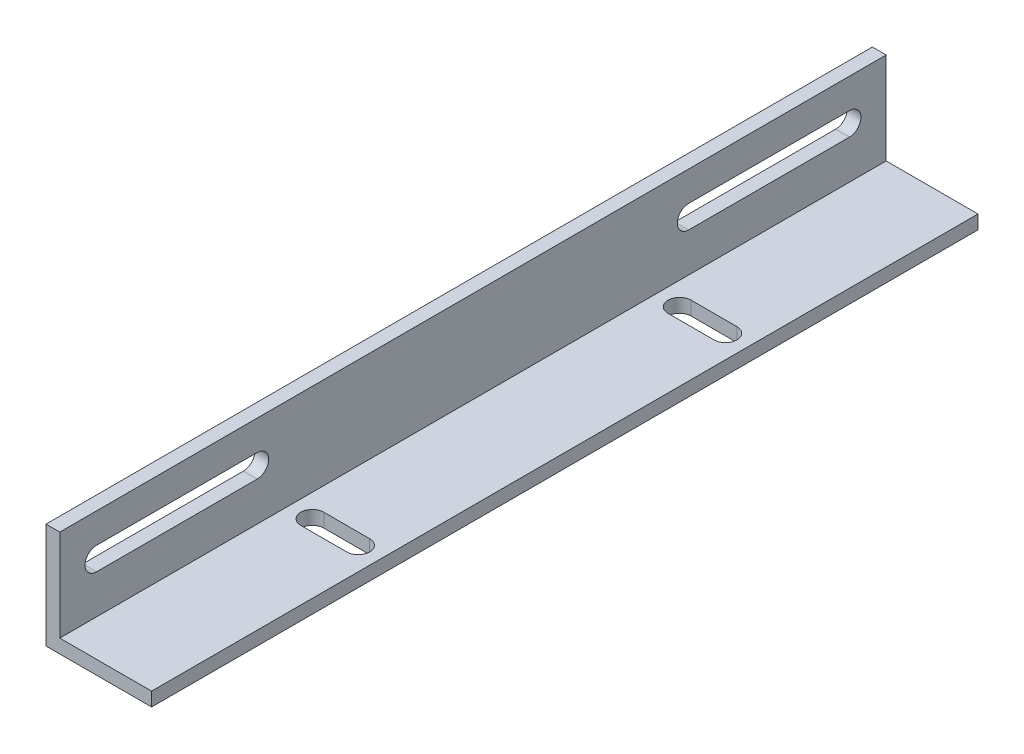
SolidWorks part; units mm, degrees
ref_plane "前视基准面" through (0, 0, 0) normal (0, 0, 1) x (1, 0, 0)
ref_plane "上视基准面" through (0, 0, 0) normal (0, 1, 0) x (1, 0, 0)
ref_plane "右视基准面" through (0, 0, 0) normal (1, 0, 0) x (0, 0, -1)
sketch "草图1" plane through (0, 0, 0) normal (0, 0, 1) x (1, 0, 0)
  line L0 (0, 0) -> (0, 23)
  line L1 (0, 23) -> (3, 23)
  line L2 (3, 23) -> (3, 3)
  line L3 (3, 3) -> (23, 3)
  line L4 (23, 3) -> (23, 0)
  line L5 (23, 0) -> (0, 0)
  dimension "D1" = 3
  dimension "D2" = 20
extrude "凸台-拉伸1" add sketch "草图1" along normal mid plane 180
sketch "草图3" plane through (3, 0, 0) normal (1, 0, 0) x (0, 0, -1)
  line L0 (-82, 14) -> (-47, 14) construction
  line L1 (-82, 16.5) -> (-47, 16.5)
  line L2 (-82, 11.5) -> (-47, 11.5)
  line L3 (-90, 3) -> (-90, 23) construction
  line L4 (-90, 23) -> (90, 23) construction
  arc A0 (-82, 16.5) -> (-82, 11.5) centre (-82, 14) ccw
  arc A1 (-47, 11.5) -> (-47, 16.5) centre (-47, 14) ccw
  point P2 (-64.5, 14)
  dimension "D3" = 2.5
  dimension "D1" = 35
  dimension "D2" = 8
  dimension "D4" = 9
extrude "切除-拉伸1" cut sketch "草图3" against normal up to next
mirror "镜向1" about plane through (0, 0, 0) normal (0, 0, 1) of "切除-拉伸1"
sketch "草图4" plane through (0, 3, 0) normal (0, 1, 0) x (1, 0, 0)
  line L0 (8, 40) -> (18, 40) construction
  line L1 (8, 42.5) -> (18, 42.5)
  line L2 (8, 37.5) -> (18, 37.5)
  line L3 (8, -40) -> (18, -40) construction
  line L4 (8, -37.5) -> (18, -37.5)
  line L5 (8, -42.5) -> (18, -42.5)
  line L6 (23, -90) -> (23, 90) construction
  arc A0 (8, 42.5) -> (8, 37.5) centre (8, 40) ccw
  arc A1 (18, 37.5) -> (18, 42.5) centre (18, 40) ccw
  arc A2 (8, -37.5) -> (8, -42.5) centre (8, -40) ccw
  arc A3 (18, -42.5) -> (18, -37.5) centre (18, -40) ccw
  point P2 (13, 40)
  point P8 (13, -40)
  dimension "D3" = 2.5
  dimension "D1" = 40
  dimension "D2" = 10
  dimension "D4" = 5
  dimension "D5" = 40
extrude "切除-拉伸2" cut sketch "草图4" against normal up to next
